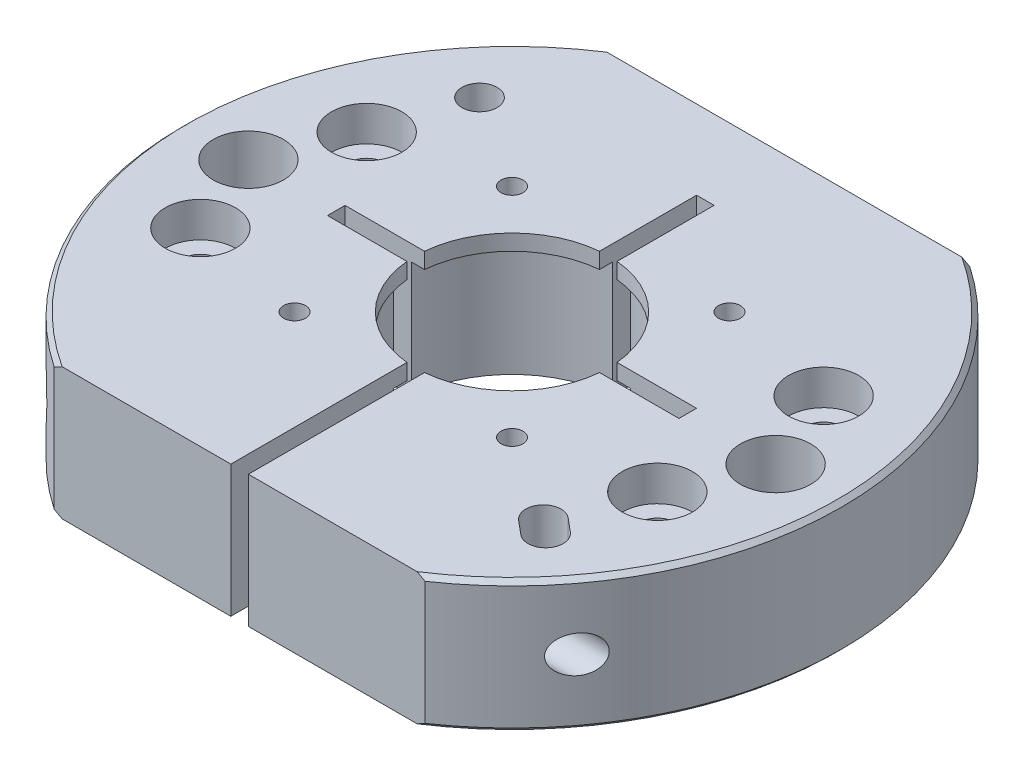
from build123d import *

# Parameters (mm, degrees)
SKETCH1_R           = 37.5
SKETCH1_R_2         = 12.5
BOSS_EXTRUDE1_DEPTH = 15
SKETCH2_R           = 4
CUT_EXTRUDE1_DEPTH  = 4
SKETCH3_R           = 2
CUT_EXTRUDE2_DEPTH  = 56.113519213
SKETCH4_W           = 40
SKETCH4_H           = 2
CUT_EXTRUDE3_DEPTH  = 16
SKETCH5_W           = 2
SKETCH5_H           = 67
CUT_EXTRUDE4_DEPTH  = 16
CHAMFER1_SIZE       = 0.5
SKETCH6_R           = 2.75
CUT_EXTRUDE5_DEPTH  = 27
SKETCH7_R           = 5.5
CUT_EXTRUDE6_DEPTH  = 27
SKETCH8_R           = 0.542778956
CUT_EXTRUDE7_DEPTH  = 27
M5_TAPPED_HOLE1_D   = 4.2
SKETCH10_R          = 4
CUT_EXTRUDE8_DEPTH  = 56.113519349
SKETCH11_W          = 70
SKETCH11_H          = 13
CUT_EXTRUDE9_DEPTH  = 56.113519349
SKETCH16_R          = 2
CUT_EXTRUDE11_DEPTH = 51.914143553
BOSS_EXTRUDE2_START = -1.8
BOSS_EXTRUDE2_DEPTH = 1.8
SKETCH19_R          = 1
CUT_EXTRUDE12_DEPTH = 5
CIRPATTERN2_COUNT   = 4


with BuildPart() as part:
    # Sketch1 → Boss-Extrude1 (new body)
    with BuildSketch(Plane(origin=(0, 0, 0), x_dir=(1, 0, 0), z_dir=(0, 1, 0))):
        with Locations(Location((0, 0, 0), (0, 0, 270))):
            Circle(SKETCH1_R)
        with Locations(Location((0, 0, 0), (0, 0, 270))):
            Circle(SKETCH1_R_2, mode=Mode.SUBTRACT)
    extrude(amount=BOSS_EXTRUDE1_DEPTH)

    # Sketch2 → Cut-Extrude1 (cut)
    with BuildSketch(Plane(origin=(0, 15, 0), x_dir=(1, 0, 0), z_dir=(0, 1, 0))):
        with Locations(Location((26, -9.463226091, 0), (0, 0, 270))):
            Circle(SKETCH2_R)
        with Locations(Location((-26, 9.463226091, 0), (0, 0, 270))):
            Circle(SKETCH2_R)
        with Locations(Location((-26, -9.463226091, 0), (0, 0, 90))):
            Circle(SKETCH2_R)
        with Locations(Location((26, 9.463226091, 0), (0, 0, 90))):
            Circle(SKETCH2_R)
    extrude(amount=-CUT_EXTRUDE1_DEPTH, mode=Mode.SUBTRACT)

    # Sketch3 → Cut-Extrude2 (cut, through all)
    with BuildSketch(Plane(origin=(0, 15, 0), x_dir=(1, 0, 0), z_dir=(0, 1, 0))):
        with Locations(Location((-26, 9.463226091, 0), (0, 0, 270))):
            Circle(SKETCH3_R)
        with Locations(Location((-26, -9.463226091, 0), (0, 0, 270))):
            Circle(SKETCH3_R)
        with Locations(Location((26, 9.463226091, 0), (0, 0, 270))):
            Circle(SKETCH3_R)
        with Locations(Location((26, -9.463226091, 0), (0, 0, 270))):
            Circle(SKETCH3_R)
    extrude(amount=-CUT_EXTRUDE2_DEPTH, mode=Mode.SUBTRACT)

    # Sketch4 → Cut-Extrude3 (cut)
    with BuildSketch(Plane(origin=(0, 15, 0), x_dir=(1, 0, 0), z_dir=(0, 1, 0))):
        Rectangle(SKETCH4_W, SKETCH4_H)
    extrude(amount=-CUT_EXTRUDE3_DEPTH, mode=Mode.SUBTRACT)

    # Sketch5 → Cut-Extrude4 (cut)
    with BuildSketch(Plane(origin=(0, 15, 0), x_dir=(1, 0, 0), z_dir=(0, 1, 0))):
        with Locations((0, -11.5)):
            Rectangle(SKETCH5_W, SKETCH5_H)
    extrude(amount=-CUT_EXTRUDE4_DEPTH, mode=Mode.SUBTRACT)

    # Chamfer1
    chamfer1_edges = [part.edges().sort_by_distance(p)[0] for p in [
        (0, 0, -37.5),
        (0, 15, -37.5),
    ]]
    chamfer(chamfer1_edges, length=CHAMFER1_SIZE)

    # Sketch6 → Cut-Extrude5 (cut)
    with BuildSketch(Plane(origin=(0, 0, 0), x_dir=(0, 0, -1), z_dir=(1, 0, 0))):
        with Locations((-22.5, 7.5)):
            Circle(SKETCH6_R)
    extrude(amount=-CUT_EXTRUDE5_DEPTH, mode=Mode.SUBTRACT)

    # Sketch7 → Cut-Extrude6 (cut)
    with BuildSketch(Plane(origin=(-8.5, 0, 0), x_dir=(0, 0, -1), z_dir=(1, 0, 0))):
        with Locations((-22.5, 7.5)):
            Circle(SKETCH7_R)
    extrude(amount=-CUT_EXTRUDE6_DEPTH, mode=Mode.SUBTRACT)

    # Sketch8 → Cut-Extrude7 (cut)
    with BuildSketch(Plane.ZY.offset(-1)):
        with Locations((22.5, 7.5)):
            Circle(SKETCH8_R)
    extrude(amount=-CUT_EXTRUDE7_DEPTH, mode=Mode.SUBTRACT)

    # M5 Tapped Hole1 (through all)
    with Locations(Plane(origin=(1, 7.5, 22.5), x_dir=(0, 0, -1), z_dir=(-1, 0, 0))):
        with Locations((0, 0)):
            Hole(M5_TAPPED_HOLE1_D / 2)

    # Sketch10 → Cut-Extrude8 (cut, through all)
    with BuildSketch(Plane(origin=(0, 15, 0), x_dir=(1, 0, 0), z_dir=(0, 1, 0))):
        with Locations(Location((-30, 0, 0), (0, 0, 270))):
            Circle(SKETCH10_R)
        with Locations(Location((30, 0, 0), (0, 0, 90))):
            Circle(SKETCH10_R)
    extrude(amount=-CUT_EXTRUDE8_DEPTH, mode=Mode.SUBTRACT)

    # Sketch11 → Cut-Extrude9 (cut, through all)
    with BuildSketch(Plane(origin=(0, 15, 0), x_dir=(1, 0, 0), z_dir=(0, 1, 0))):
        with Locations((0, -37.5)):
            Rectangle(SKETCH11_W, SKETCH11_H)
        with Locations((0, 37.5)):
            Rectangle(SKETCH11_W, SKETCH11_H)
    extrude(amount=-CUT_EXTRUDE9_DEPTH, mode=Mode.SUBTRACT)

    # Sketch16 → Cut-Extrude11 (cut, through all)
    with BuildSketch(Plane.XZ):
        with Locations(Location((-22.981333294, -19.283628291, 0), (0, 0, 270))):
            Circle(SKETCH16_R)
        with BuildLine():
            Line((25.032952956, 18.394327014), (23.50086407, 17.108751795))
            ThreePointArc((23.50086407, 17.108751795), (20.683199964, 17.355265462), (20.929713631, 20.172929567))
            Line((20.929713631, 20.172929567), (22.461802517, 21.458504787))
            ThreePointArc((22.461802517, 21.458504787), (25.279466623, 21.21199112), (25.032952956, 18.394327014))
        make_face()
    extrude(amount=-CUT_EXTRUDE11_DEPTH, mode=Mode.SUBTRACT)

    # Sketch17 → Boss-Extrude2 (add)
    with BuildSketch(Plane(origin=(0, 15, 0), x_dir=(1, 0, 0), z_dir=(0, 1, 0)).offset(BOSS_EXTRUDE2_START)):
        with BuildLine():
            Line((1, 12.459935794), (1, 10.95445115))
            ThreePointArc((1, 10.95445115), (7.778174593, 7.778174593), (10.95445115, 1))
            Line((10.95445115, 1), (12.459935794, 1))
            ThreePointArc((12.459935794, 1), (8.838834765, 8.838834765), (1, 12.459935794))
        make_face()
        with BuildLine():
            Line((-1, 12.459935794), (-1, 10.95445115))
            ThreePointArc((-1, 10.95445115), (-7.778174593, 7.778174593), (-10.95445115, 1))
            Line((-10.95445115, 1), (-12.459935794, 1))
            ThreePointArc((-12.459935794, 1), (-8.838834765, 8.838834765), (-1, 12.459935794))
        make_face()
        with BuildLine():
            Line((12.459935794, -1), (10.95445115, -1))
            ThreePointArc((10.95445115, -1), (7.778174593, -7.778174593), (1, -10.95445115))
            Line((1, -10.95445115), (1, -12.459935794))
            ThreePointArc((1, -12.459935794), (8.838834765, -8.838834765), (12.459935794, -1))
        make_face()
        with BuildLine():
            Line((-12.459935794, -1), (-10.95445115, -1))
            ThreePointArc((-10.95445115, -1), (-7.778174593, -7.778174593), (-1, -10.95445115))
            Line((-1, -10.95445115), (-1, -12.459935794))
            ThreePointArc((-1, -12.459935794), (-8.838834765, -8.838834765), (-12.459935794, -1))
        make_face()
    extrude(amount=BOSS_EXTRUDE2_DEPTH)

    # Sketch19 → Cut-Extrude12 (cut)
    with BuildSketch(Plane(origin=(0, 15, 0), x_dir=(1, 0, 0), z_dir=(0, 1, 0))):
        with Locations(Location((-12.374368671, 12.374368671, 0), (0, 0, 270))):
            Circle(SKETCH19_R)
    extrude(amount=-CUT_EXTRUDE12_DEPTH, mode=Mode.SUBTRACT)

    # Sketch20 → M3 Tapped Hole2 (revolve, cut)
    with BuildSketch(Plane(origin=(-12.374368671, 15, -12.374368671), x_dir=(0, 0, 1), z_dir=(1, 0, 0))):
        Polygon((0, 0), (0, 7.251075774), (1.25, 6.5), (1.25, 0), align=None)
    m3_tapped_hole2 = revolve(axis=Axis((-12.374368671, 21.35, -12.374368671), (0, -1, 0)), mode=Mode.SUBTRACT)

    # CirPattern2: M3 Tapped Hole2 ×4 about axis
    cirpattern2_axis = Axis((0, 0, 0), (0, 1, 0))
    for i in range(1, CIRPATTERN2_COUNT):
        add(m3_tapped_hole2.rotate(cirpattern2_axis, i * 360 / CIRPATTERN2_COUNT), mode=Mode.SUBTRACT)


solid = part.part
